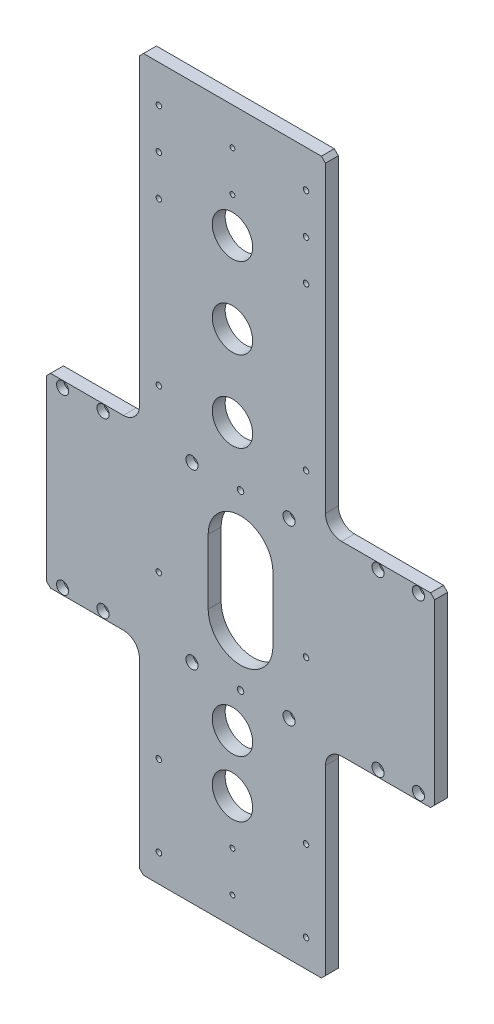
from build123d import *

# Parameters (mm, degrees)
SKETCH_1_W                = 230
SKETCH_1_H                = 400
SKETCH_1_W_2              = 480
SKETCH_1_H_2              = 230
SKETCH_1_H_3              = 250
EXTRUDE_1_DEPTH           = 16
FILLET_1_R                = 20
HOLE_WIZARD_1_D           = 9
HOLE_WIZARD_1_CBORE_D     = 15
HOLE_WIZARD_1_CBORE_DEPTH = 9
MM_1_D                    = 8
HOLE_WIZARD_M8_1_D        = 6.8
HOLE_WIZARD_M8_1_DEPTH    = 22.25
HOLE_WIZARD_M8_1_TIP      = 2.042926105
CHAMFER_1_SIZE            = 5
SKETCH_8_R                = 25
CUT_EXTRUDE_1_DEPTH       = 569.402146372
MM_4_D                    = 6


with BuildPart() as part:
    # 草图1 → 凸台-拉伸1 (new body)
    with BuildSketch(Plane.XY):
        with Locations((-10, 315)):
            Rectangle(SKETCH_1_W, SKETCH_1_H)
        Rectangle(SKETCH_1_W_2, SKETCH_1_H_2)
        with Locations((-10, -240)):
            Rectangle(SKETCH_1_W, SKETCH_1_H_3)
    extrude(amount=EXTRUDE_1_DEPTH)

    # 圆角1
    fillet_1_edges = [part.edges().sort_by_distance(p)[0] for p in [
        (105, 115, 8),
        (105, -115, 8),
        (-125, -115, 8),
        (-125, 115, 8),
    ]]
    fillet(fillet_1_edges, radius=FILLET_1_R)

    # 打孔尺寸(%根据)内六角圆柱头螺钉的类型1 (through all)
    with Locations(Plane.XY.offset(16)):
        with Locations((60, -107), (220, 107), (-220, -107), (-220, 107), (220, -107), (-170, 107), (-170, -107), (170, 107), (170, -107), (-60, 107), (-60, -107), (60, 107)):
            CounterBoreHole(HOLE_WIZARD_1_D / 2, HOLE_WIZARD_1_CBORE_D / 2, HOLE_WIZARD_1_CBORE_DEPTH)

    # 大小mm 暗销孔1 (through all)
    with Locations(Plane.XY.offset(16)):
        with Locations((0, 107), (0, -107)):
            Hole(MM_1_D / 2)

    # M8 螺纹孔1
    with Locations(Plane.XY.offset(16)):
        with Locations((81, 469), (-101, 469), (-101, 169), (-101, 369), (-101, 419), (-101, -31), (-101, -231), (-101, -331), (81, -331), (81, -231), (81, -31), (81, 419), (81, 369), (81, 169)):
            Hole(HOLE_WIZARD_M8_1_D / 2, depth=HOLE_WIZARD_M8_1_DEPTH)
            with Locations((0, 0, -(HOLE_WIZARD_M8_1_DEPTH + HOLE_WIZARD_M8_1_TIP / 2))):  # 118° drill point
                Cone(0, HOLE_WIZARD_M8_1_D / 2, HOLE_WIZARD_M8_1_TIP, mode=Mode.SUBTRACT)

    # 倒角1
    chamfer_1_edges = [part.edges().sort_by_distance(p)[0] for p in [
        (240, 115, 8),
        (240, -115, 8),
        (105, -365, 8),
        (-125, -365, 8),
        (-240, -115, 8),
        (-240, 115, 8),
        (-125, 515, 8),
        (105, 515, 8),
    ]]
    chamfer(chamfer_1_edges, length=CHAMFER_1_SIZE)

    # 草图8 → 切除-拉伸1 (cut, through all)
    with BuildSketch(Plane.XY.offset(16)):
        with Locations((-10, 375)):
            Circle(SKETCH_8_R)
        with Locations((-10, -155)):
            Circle(SKETCH_8_R)
        with Locations((-10, -225)):
            Circle(SKETCH_8_R)
        with Locations((-10, 275)):
            Circle(SKETCH_8_R)
        with Locations((-10, 175)):
            Circle(SKETCH_8_R)
        with BuildLine():
            Line((-40, -40), (-40, 40))
            ThreePointArc((-40, 40), (0, 80), (40, 40))
            Line((40, 40), (40, -40))
            ThreePointArc((40, -40), (0, -80), (-40, -40))
        make_face()
    extrude(amount=-CUT_EXTRUDE_1_DEPTH, mode=Mode.SUBTRACT)

    # 大小mm 暗销孔4 (through all)
    with Locations(Plane.XY.offset(16)):
        with Locations((-10, 419), (-10, -331), (-10, -281), (-10, 469)):
            Hole(MM_4_D / 2)


solid = part.part
